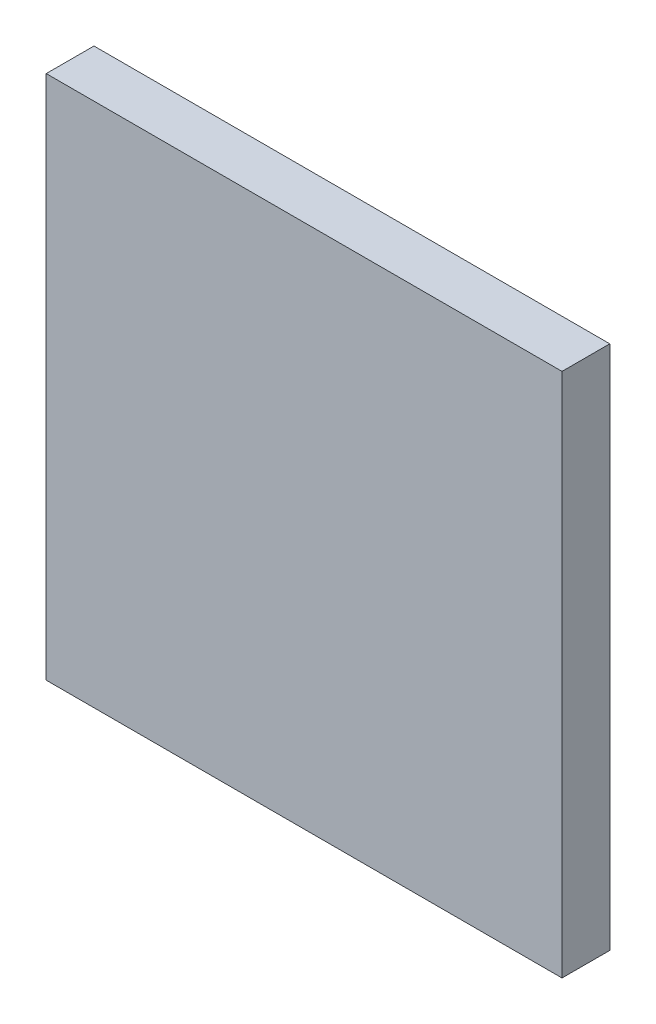
from build123d import *

# Parameters (mm, degrees)
SKETCH_1_W      = 108
SKETCH_1_H      = 110
EXTRUDE_1_DEPTH = 5


with BuildPart() as part:
    # 草图1 → 凸台-拉伸1 (new, symmetric)
    with BuildSketch(Plane.XY):
        Rectangle(SKETCH_1_W, SKETCH_1_H)
    extrude(amount=EXTRUDE_1_DEPTH, both=True)


solid = part.part
